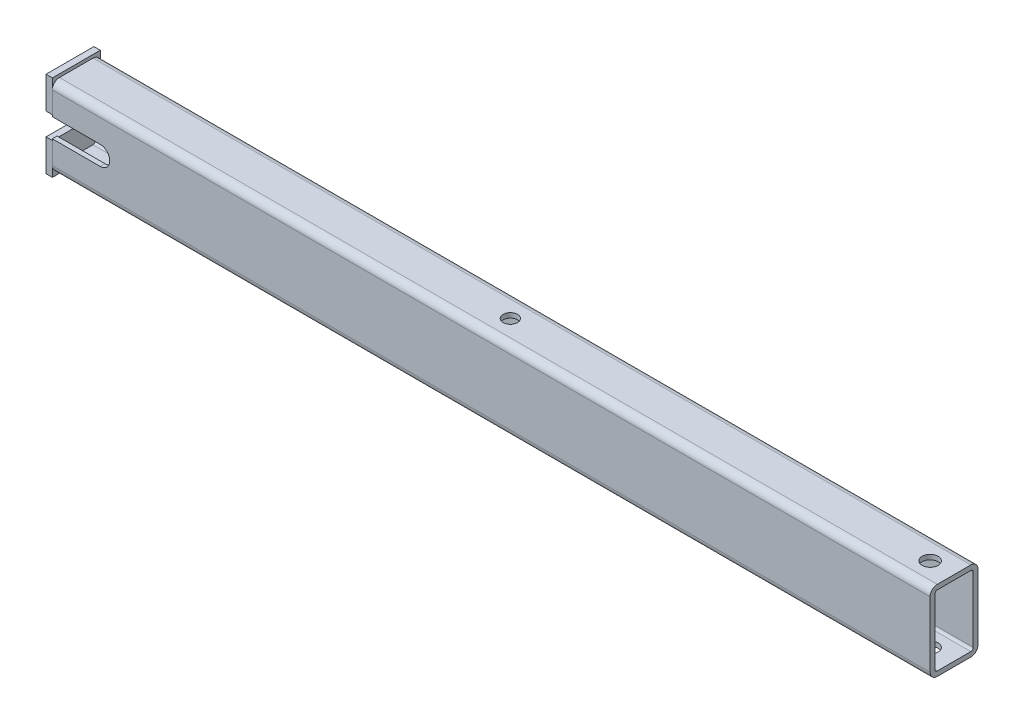
SolidWorks part; units mm, degrees
material "Q235B"
ref_plane "Front" through (0, 0, 0) normal (0, 0, 1) x (1, 0, 0)
ref_plane "Top" through (0, 0, 0) normal (0, 1, 0) x (1, 0, 0)
ref_plane "Right" through (0, 0, 0) normal (1, 0, 0) x (0, 0, -1)
sketch "草图1" plane through (0, 0, 0) normal (0, 0, 1) x (1, 0, 0)
  line L0 (-232.2108, 0) -> (317.7892, 0)
  dimension "D1" = 550
other "Structural Member2"
ref_plane "Plane2" through (-232.2108, 0, 0) normal (1, 0, 0) x (0, 1, 0)
sketch "Sketch1" plane through (-232.2108, 0, 0) normal (1, 0, 0) x (0, 1, 0)
  line L0 (-20.5, -12) -> (20.5, -12)
  line L1 (-22, -10.5) -> (-22, 10.5)
  line L2 (20.5, 12) -> (-20.5, 12)
  line L3 (22, 10.5) -> (22, -10.5)
  line L4 (-20.5, -15) -> (20.5, -15)
  line L5 (-25, -10.5) -> (-25, 10.5)
  line L6 (20.5, 15) -> (-20.5, 15)
  line L7 (25, 10.5) -> (25, -10.5)
  arc A0 (25, 10.5) -> (20.5, 15) centre (20.5, 10.5) ccw
  arc A1 (20.5, -15) -> (25, -10.5) centre (20.5, -10.5) ccw
  arc A2 (-25, -10.5) -> (-20.5, -15) centre (-20.5, -10.5) ccw
  arc A3 (-20.5, 15) -> (-25, 10.5) centre (-20.5, 10.5) ccw
  arc A4 (-20.5, 12) -> (-22, 10.5) centre (-20.5, 10.5) ccw
  arc A5 (22, 10.5) -> (20.5, 12) centre (20.5, 10.5) ccw
  arc A6 (20.5, -12) -> (22, -10.5) centre (20.5, -10.5) ccw
  arc A7 (-22, -10.5) -> (-20.5, -12) centre (-20.5, -10.5) ccw
  point P0 (-25, 0)
  point P1 (25, 0)
  point P2 (0, 15)
  point P3 (0, -15)
  point P4 (0, 0)
  point P5 (-25, -15)
  point P6 (25, -15)
  point P7 (25, 15)
  point P8 (-25, 15)
  point P33 (0, 7.5)
  point P35 (0, -7.5)
  point P36 (12.5, 0)
  point P37 (-12.5, 0)
  point P38 (0, 12)
  point P39 (-22, 0)
  point P40 (22, 0)
  point P41 (0, -12)
  point P42 (-12.5, -7.5)
  point P43 (12.5, -7.5)
  point P44 (12.5, 7.5)
  point P45 (-12.5, 7.5)
  point P46 (-12.5, 12)
  point P47 (-12.5, 15)
  point P48 (-22, 7.5)
  point P49 (-25, 7.5)
  point P50 (22, 7.5)
  point P51 (25, 7.5)
  point P52 (12.5, 12)
  point P53 (12.5, 15)
  point P54 (22, -7.5)
  point P55 (25, -7.5)
  point P56 (12.5, -12)
  point P57 (12.5, -15)
  point P58 (-12.5, -12)
  point P59 (-12.5, -15)
  point P60 (-22, -7.5)
  point P61 (-25, -7.5)
  point P62 (0, 0)
sketch "Sketch4" plane through (0, 0, 15) normal (0, 0, 1) x (1, 0, 0)
  line L0 (-232.2108, 0) -> (-202.2108, 0) construction
  line L1 (-232.2108, 20.5) -> (-232.2108, -20.5) construction
  line L2 (-232.2108, 0) -> (317.7892, 0) construction
  line L3 (-232.2108, 6) -> (-202.2108, 6)
  line L4 (-232.2108, -6) -> (-202.2108, -6)
  arc A0 (-232.2108, 6) -> (-232.2108, -6) centre (-232.2108, 0) ccw
  arc A1 (-202.2108, -6) -> (-202.2108, 6) centre (-202.2108, 0) ccw
  point P6 (-217.2108, 0)
extrude "Cut-Extrude1" cut sketch "Sketch4" against normal through all
sketch "Sketch5" plane through (0, -25, 0) normal (0, -1, 0) x (-1, 0, 0)
  line L0 (-302.7892, 65) -> (-302.7892, -36.6281) construction
  circle A0 centre (-302.7892, 0) radius 5
  dimension "D1" = 10
extrude "Cut-Extrude2" cut sketch "Sketch5" against normal blind 50
sketch "Sketch6" plane through (0, 25, 0) normal (0, 1, 0) x (1, 0, 0)
  circle A0 centre (39.7892, 0) radius 4.5
  dimension "D1" = 9
extrude "Cut-Extrude3" cut sketch "Sketch6" against normal through all
sketch "Sketch7" plane through (-232.2108, 0, 0) normal (-1, 0, 0) x (0, 0, 1)
  line L0 (-15, 6) -> (-12, 6) construction
  line L1 (14.9388, 7) -> (-15.0612, 7)
  line L2 (14.9388, 7) -> (14.9388, 27)
  line L3 (14.9388, 27) -> (-15.0612, 27)
  line L4 (-15.0612, 7) -> (-15.0612, 27)
  line L5 (-0.0612, 27) -> (-0.0612, 7) construction
  line L6 (14.9388, 17) -> (-15.0612, 17) construction
  point P0 (-0.0612, 17)
  dimension "D1" = 30
  dimension "D2" = 20
  dimension "D3" = 1
extrude "Boss-Extrude1" add sketch "Sketch7" along normal blind 4 separate body
mirror "Mirror2" about plane through (0, 0, 0) normal (0, 1, 0) of bodies 106
equation "\"零件重量\"= IIF ( \"SW-质量\" > 100 , int ( \"SW-质量\" ) , \"SW-质量\" )"
equation "\"D4@Sketch1\"=\"A@Sketch1\"/4"
equation "\"D2@Sketch1\"= \"B@Sketch1\" / 4"
equation "\"D5@Sketch1\"=\"A@Sketch1\" / 4"
equation "\"D3@Sketch1\"= \"B@Sketch1\" / 4"
